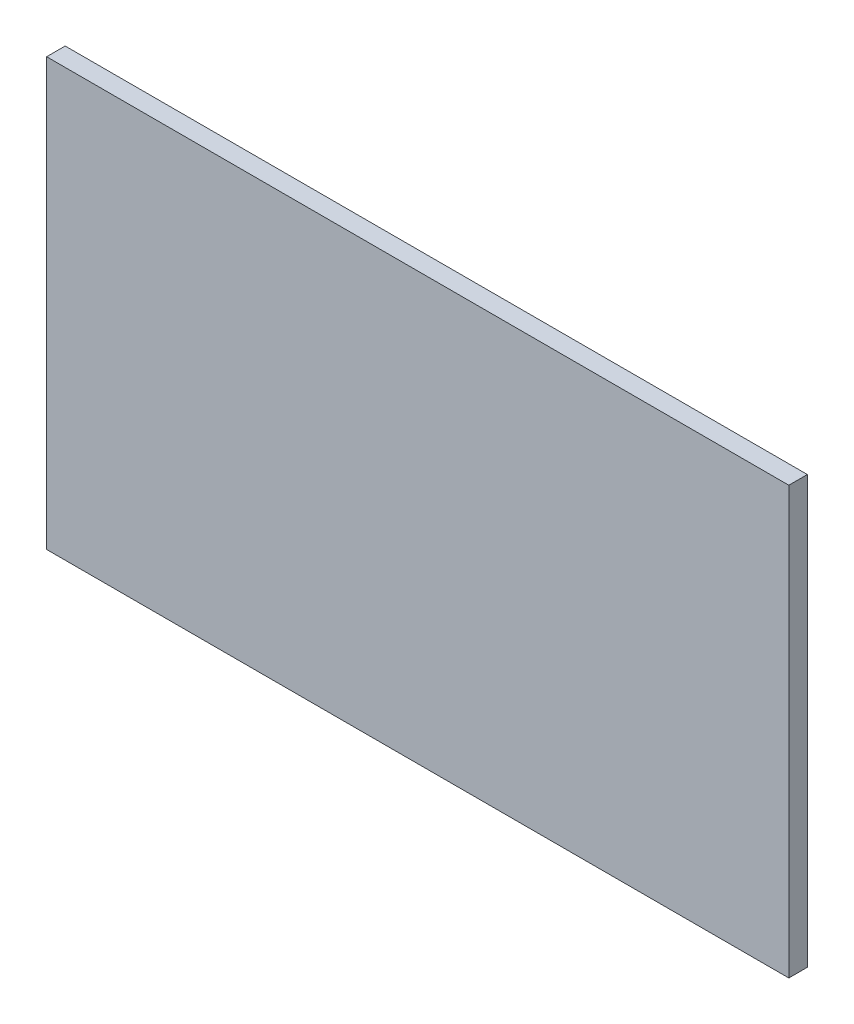
from build123d import *

# Parameters (mm, degrees)
SKETCH1_W           = 400
SKETCH1_H           = 230
BOSS_EXTRUDE1_DEPTH = 10


with BuildPart() as part:
    # Sketch1 → Boss-Extrude1 (new body)
    with BuildSketch(Plane.XY):
        Rectangle(SKETCH1_W, SKETCH1_H)
    extrude(amount=BOSS_EXTRUDE1_DEPTH)


solid = part.part
